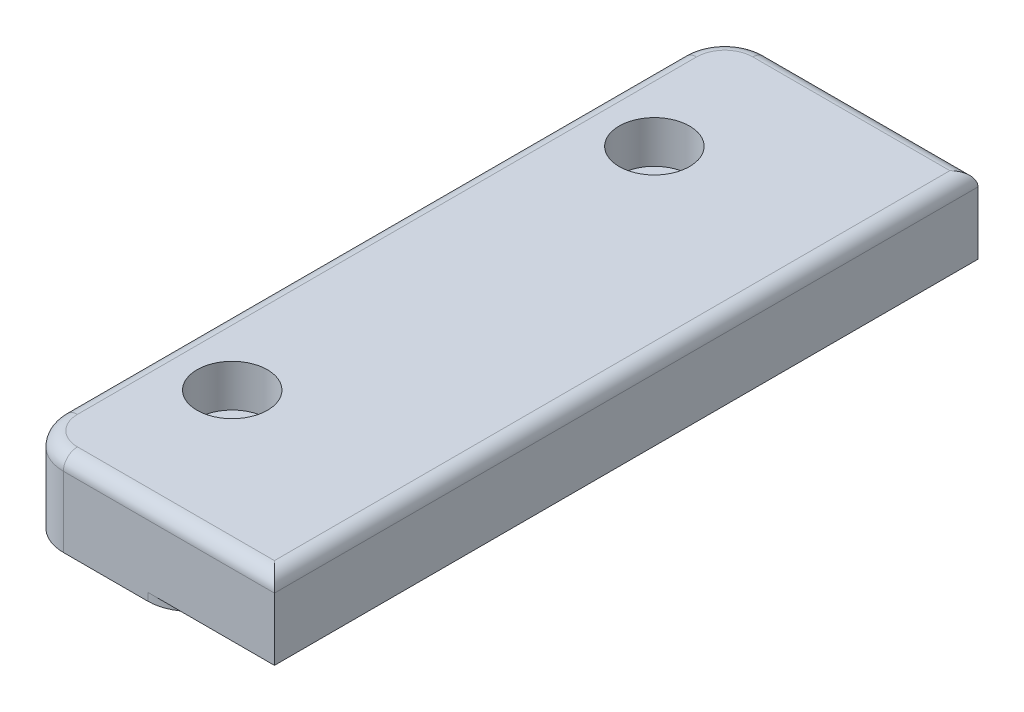
SolidWorks part; units mm, degrees
ref_plane "Front Plane" through (0, 0, 0) normal (0, 0, 1) x (1, 0, 0)
ref_plane "Top Plane" through (0, 0, 0) normal (0, 1, 0) x (1, 0, 0)
ref_plane "Right Plane" through (0, 0, 0) normal (1, 0, 0) x (0, 0, -1)
other "Configuration Table"
sketch "Sketch1" plane through (0, 0, 0) normal (0, 0, 1) x (1, 0, 0)
  line L0 (-30.7895, 0) -> (33.6316, 0) construction
  line L1 (-4.7368, 0) -> (-4.7368, 6)
  line L2 (-4.7368, 6) -> (13.2632, 6)
  line L3 (13.2632, 6) -> (13.2632, 0.55)
  line L4 (13.2632, 0.55) -> (7.2632, 0.55)
  line L5 (7.2632, 0.55) -> (7.2632, 0)
  line L6 (7.2632, 0) -> (-4.7368, 0)
  dimension "D1" = 18
  dimension "D2" = 6
  dimension "D3" = 0.55
  dimension "D4" = 12
extrude "Boss-Extrude1" add sketch "Sketch1" along normal blind 50
fillet "Fillet1" radius 3 1 edges at (7.2632, 0.275, 50)
sketch "Sketch3" plane through (0, 6, 0) normal (0, 1, 0) x (1, 0, 0)
  line L3 (-4.7368, -50) -> (-4.7368, 0) construction
  circle A0 centre (0.2632, -10) radius 2.5
  circle A1 centre (0.2632, -40) radius 2.5
  dimension "D2" = 5
  dimension "D3" = 5
  dimension "D1" = 30
  dimension "D5" = 5
  dimension "D6" = 5
extrude "Cut-Extrude1" cut sketch "Sketch3" against normal blind 3
sketch "Sketch4" plane through (0, 3, 0) normal (0, 1, 0) x (1, 0, 0)
  circle A0 centre (0.2632, -40) radius 1.5
  dimension "D1" = 3
extrude "Cut-Extrude2" cut sketch "Sketch4" against normal through all
sketch "Sketch5" plane through (0, 3, 0) normal (0, 1, 0) x (1, 0, 0)
  circle A0 centre (0.2632, -10) radius 1.5
  dimension "D1" = 3
extrude "Cut-Extrude3" cut sketch "Sketch5" against normal through all
fillet "Fillet5" radius 3 1 edges at (7.2632, 0.275, 0)
fillet "Fillet6" radius 3 2 edges at (-4.7368, 3, 0) (-4.7368, 3, 50)
fillet "Fillet7" radius 1 6 edges at (5.7632, 6, 50) (-3.8582, 6, 49.1213) (-4.7368, 6, 25) (-3.8582, 6, 0.8787) (5.7632, 6, 0) (13.2632, 6, 25)
sketch "Sketch6" plane through (0, 6, 0) normal (0, 1, 0) x (1, 0, 0)
  line L0 (-4.7368, -47) -> (-4.7368, -3) construction
  line L1 (-4.7368, -47) -> (-4.7368, -3)
  line L2 (7.2632, -47) -> (7.2632, -3) construction
  line L3 (7.2632, -47) -> (7.2632, -3)
  line L4 (-1.7368, -49) -> (12.2632, -49)
  line L5 (12.2632, -49) -> (12.2632, -1)
  line L6 (12.2632, -1) -> (-1.7368, -1)
  line L7 (-3.7368, -3) -> (-3.7368, -47)
  line L8 (-1.7368, -49) -> (12.2632, -49)
  line L9 (12.2632, -49) -> (12.2632, -1)
  line L10 (12.2632, -1) -> (-1.7368, -1)
  line L11 (-3.7368, -3) -> (-3.7368, -47)
  arc A2 (-3.7368, -47) -> (-1.7368, -49) centre (-1.7368, -47) ccw
  arc A3 (-1.7368, -1) -> (-3.7368, -3) centre (-1.7368, -3) ccw
  arc A4 (-3.7368, -47) -> (-1.7368, -49) centre (-1.7368, -47) ccw
  arc A5 (-1.7368, -1) -> (-3.7368, -3) centre (-1.7368, -3) ccw
  dimension "D1" = 0
